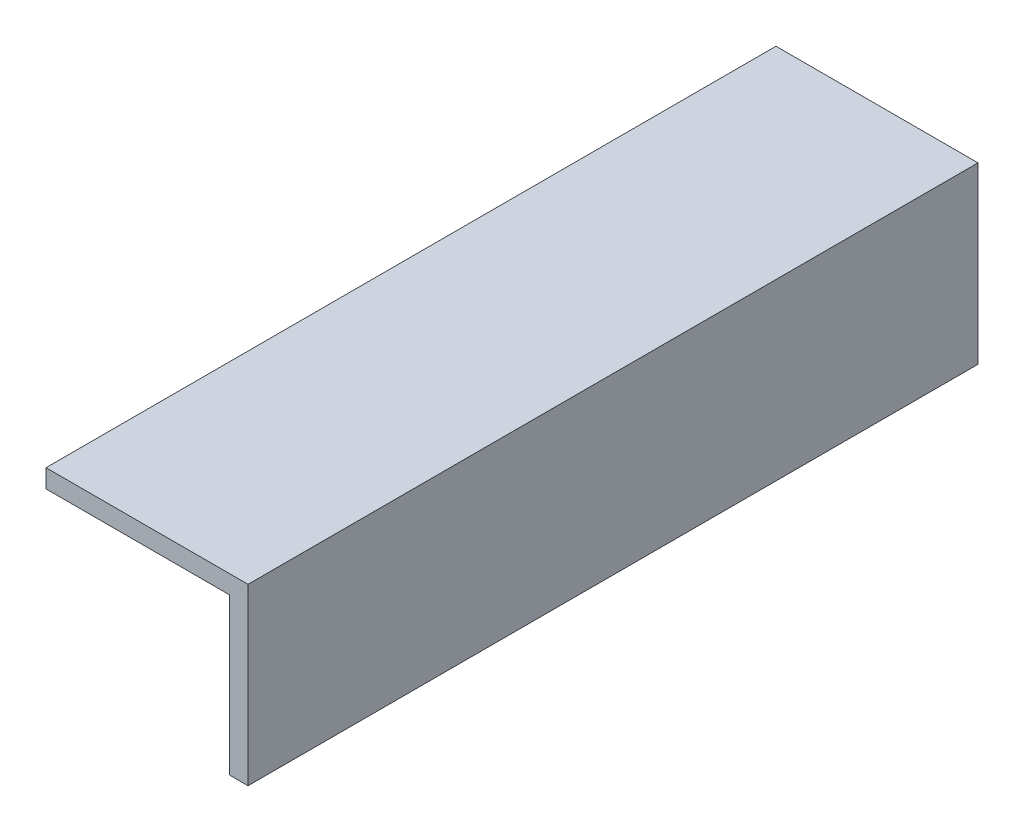
SolidWorks part; units mm, degrees
ref_plane "前视基准面" through (0, 0, 0) normal (0, 0, 1) x (1, 0, 0)
ref_plane "上视基准面" through (0, 0, 0) normal (0, 1, 0) x (1, 0, 0)
ref_plane "右视基准面" through (0, 0, 0) normal (1, 0, 0) x (0, 0, -1)
sketch "草图1" plane through (0, 0, 0) normal (0, 0, 1) x (1, 0, 0)
  line L0 (0, 0) -> (0, 60)
  line L1 (0, 60) -> (-80, 60)
  line L2 (8, 0) -> (8, 68)
  line L3 (8, 68) -> (-80, 68)
  line L4 (-80, 60) -> (-80, 68)
  line L5 (0, 0) -> (8, 0)
  dimension "D1" = 8
extrude "凸台-拉伸1" add sketch "草图1" along normal blind 300
sketch "草图2" plane through (0, 0, 300) normal (0, 0, 1) x (1, 0, 0)
  line L12 (0, 0) -> (8, 0)
  line L13 (8, 0) -> (8, 68)
  line L14 (8, 68) -> (-80, 68)
  line L15 (-80, 68) -> (-80, 60)
  line L16 (-80, 60) -> (0, 60)
  line L17 (0, 60) -> (0, 0)
  line L18 (0, 0) -> (8, 0)
  line L19 (8, 0) -> (8, 68)
  line L20 (8, 68) -> (-80, 68)
  line L21 (-80, 68) -> (-80, 60)
  line L22 (-80, 60) -> (0, 60)
  line L23 (0, 60) -> (0, 0)
  dimension "D1" = 0
extrude "凸台-拉伸2" add sketch "草图2" along normal blind 10
sketch "草图4" plane through (0, 0, 0) normal (0, 0, -1) x (-1, 0, 0)
  line L12 (-8, 0) -> (0, 0)
  line L13 (0, 0) -> (0, 60)
  line L14 (0, 60) -> (80, 60)
  line L15 (80, 60) -> (80, 68)
  line L16 (80, 68) -> (-8, 68)
  line L17 (-8, 68) -> (-8, 0)
  line L18 (-8, 0) -> (0, 0)
  line L19 (0, 0) -> (0, 60)
  line L20 (0, 60) -> (80, 60)
  line L21 (80, 60) -> (80, 68)
  line L22 (80, 68) -> (-8, 68)
  line L23 (-8, 68) -> (-8, 0)
  dimension "D1" = 0
extrude "凸台-拉伸3" add sketch "草图4" along normal blind 8
sketch "草图5" plane through (0, 0, 0) normal (0, -1, 0) x (1, 0, 0)
  line L8 (0, 310) -> (0, -8)
  line L9 (0, -8) -> (8, -8)
  line L10 (8, -8) -> (8, 310)
  line L11 (8, 310) -> (0, 310)
  line L12 (0, 310) -> (0, -8)
  line L13 (0, -8) -> (8, -8)
  line L14 (8, -8) -> (8, 310)
  line L15 (8, 310) -> (0, 310)
  dimension "D1" = 0
extrude "凸台-拉伸4" add sketch "草图5" along normal blind 8
